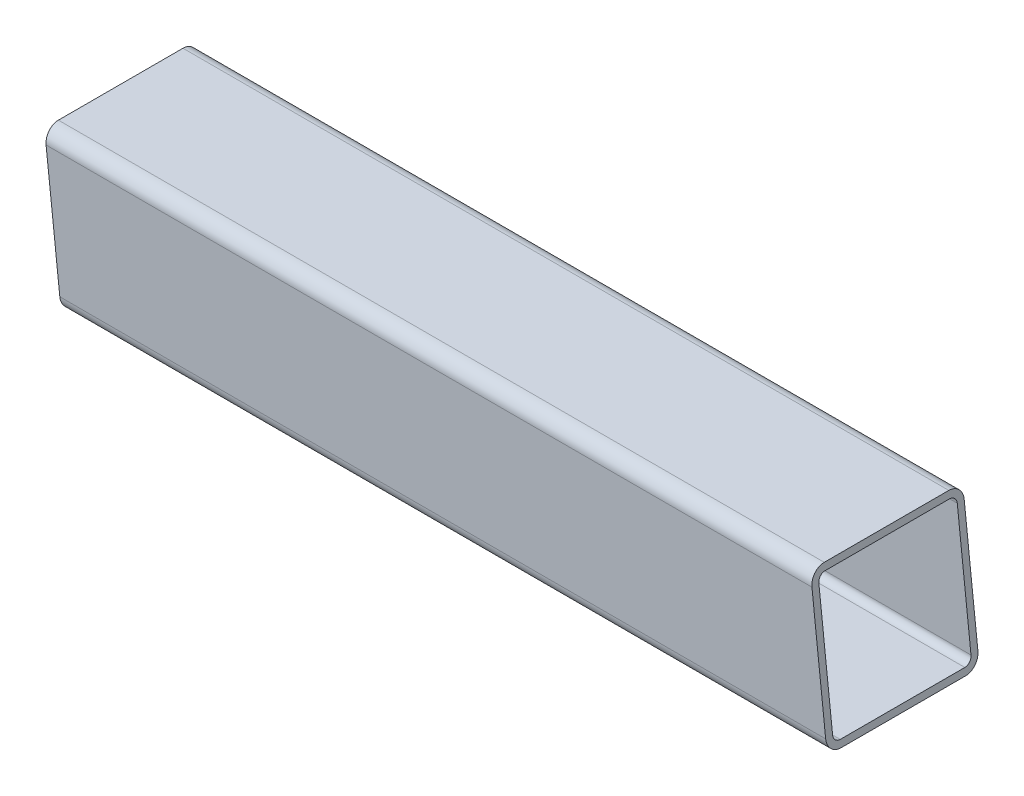
from build123d import *

# Parameters (mm, degrees)
F_110_X_110_X_5_1_DEPTH = 600
CUT_EXTRUDE_1_REACH     = 614.474


with BuildPart() as part:
    # Sketch1 → 方形管 110 X 110 X 5(1) (new body)
    with BuildSketch(Plane(origin=(0, 0, 0), x_dir=(0, 0, -1), z_dir=(1, 0, 0))):
        with BuildLine():
            Line((-45, -55), (45, -55))
            ThreePointArc((45, -55), (52.071067812, -52.071067812), (55, -45))
            Line((55, -45), (55, 45))
            ThreePointArc((55, 45), (52.071067812, 52.071067812), (45, 55))
            Line((45, 55), (-45, 55))
            ThreePointArc((-45, 55), (-52.071067812, 52.071067812), (-55, 45))
            Line((-55, 45), (-55, -45))
            ThreePointArc((-55, -45), (-52.071067812, -52.071067812), (-45, -55))
        make_face()
        with BuildLine():
            Line((-45, -50), (45, -50))
            ThreePointArc((45, -50), (48.535533906, -48.535533906), (50, -45))
            Line((50, -45), (50, 45))
            ThreePointArc((50, 45), (48.535533906, 48.535533906), (45, 50))
            Line((45, 50), (-45, 50))
            ThreePointArc((-45, 50), (-48.535533906, 48.535533906), (-50, 45))
            Line((-50, 45), (-50, -45))
            ThreePointArc((-50, -45), (-48.535533906, -48.535533906), (-45, -50))
        make_face(mode=Mode.SUBTRACT)
    extrude(amount=F_110_X_110_X_5_1_DEPTH)

    # 切除-拉伸1: up to this face of the body (flat: up to its plane)
    cut_extrude_1_end = Plane(part.part.faces().sort_by_distance((300, 0, -55))[0])
    # 草图2 → 切除-拉伸1 (cut, up to the picked face)
    with BuildSketch(Plane.XY.offset(55), mode=Mode.PRIVATE) as cut_extrude_1_sk1:
        Polygon((0, 148.583103171), (22.456015583, -55), (0, -55), align=None)
    cut_extrude_1_tool1 = split(extrude(cut_extrude_1_sk1.sketch, amount=-CUT_EXTRUDE_1_REACH, mode=Mode.PRIVATE), bisect_by=cut_extrude_1_end, keep=Keep.BOTH, mode=Mode.PRIVATE)
    # 草图2 → 切除-拉伸1 (cut, up to the picked face)
    with BuildSketch(Plane.XY.offset(55), mode=Mode.PRIVATE) as cut_extrude_1_sk2:
        Polygon((600, -274.46804857), (563.658380693, 55), (600, 55), align=None)
    cut_extrude_1_tool2 = split(extrude(cut_extrude_1_sk2.sketch, amount=-CUT_EXTRUDE_1_REACH, mode=Mode.PRIVATE), bisect_by=cut_extrude_1_end, keep=Keep.BOTH, mode=Mode.PRIVATE)
    add(cut_extrude_1_tool1.solids().sort_by(Axis((7.485339, 12.861034, 55), (0, 0, -1)))[0], mode=Mode.SUBTRACT)
    add(cut_extrude_1_tool2.solids().sort_by(Axis((587.886127, -54.822683, 55), (0, 0, -1)))[0], mode=Mode.SUBTRACT)


solid = part.part
